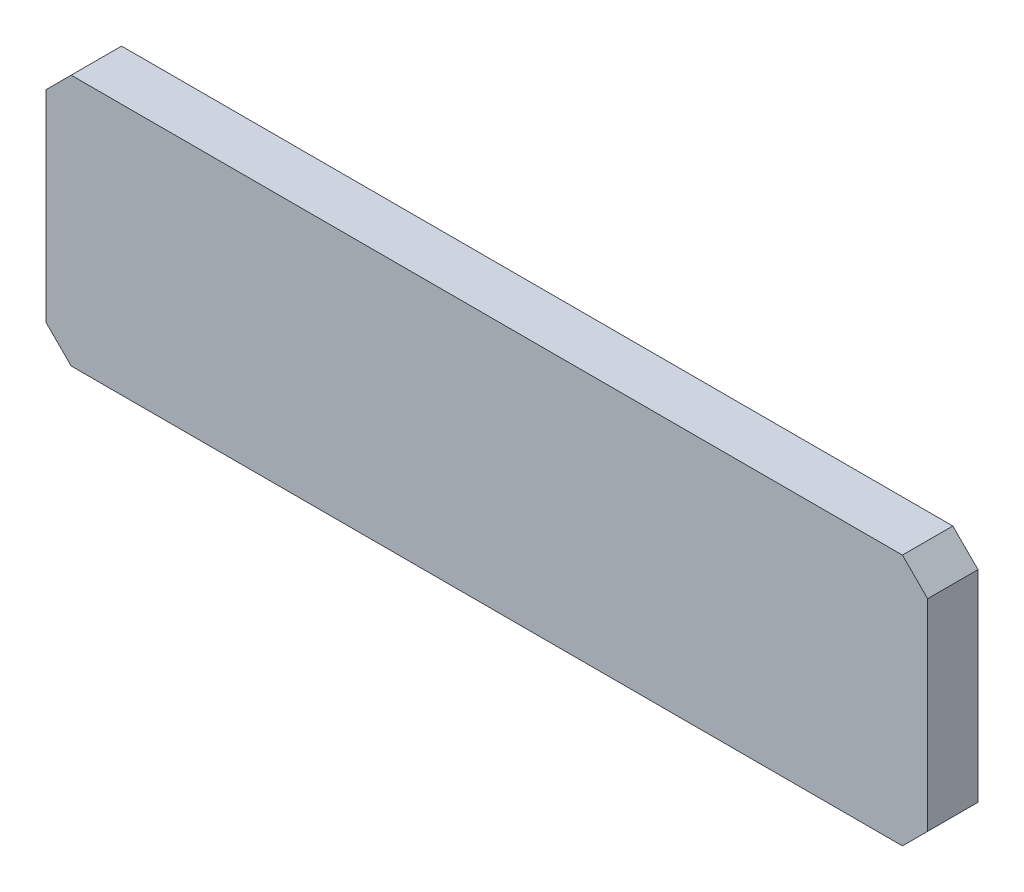
from build123d import *

# Parameters (mm, degrees)
SKETCH_1_W      = 700
SKETCH_1_H      = 200
EXTRUDE_1_DEPTH = 40
CHAMFER_1_SIZE  = 20


with BuildPart() as part:
    # 草图1 → 凸台-拉伸1 (new body)
    with BuildSketch(Plane.XY):
        Rectangle(SKETCH_1_W, SKETCH_1_H)
    extrude(amount=EXTRUDE_1_DEPTH)

    # 倒角1
    chamfer_1_edges = [part.edges().sort_by_distance(p)[0] for p in [
        (350, -100, 20),
        (-350, -100, 20),
        (-350, 100, 20),
        (350, 100, 20),
    ]]
    chamfer(chamfer_1_edges, length=CHAMFER_1_SIZE)


solid = part.part
